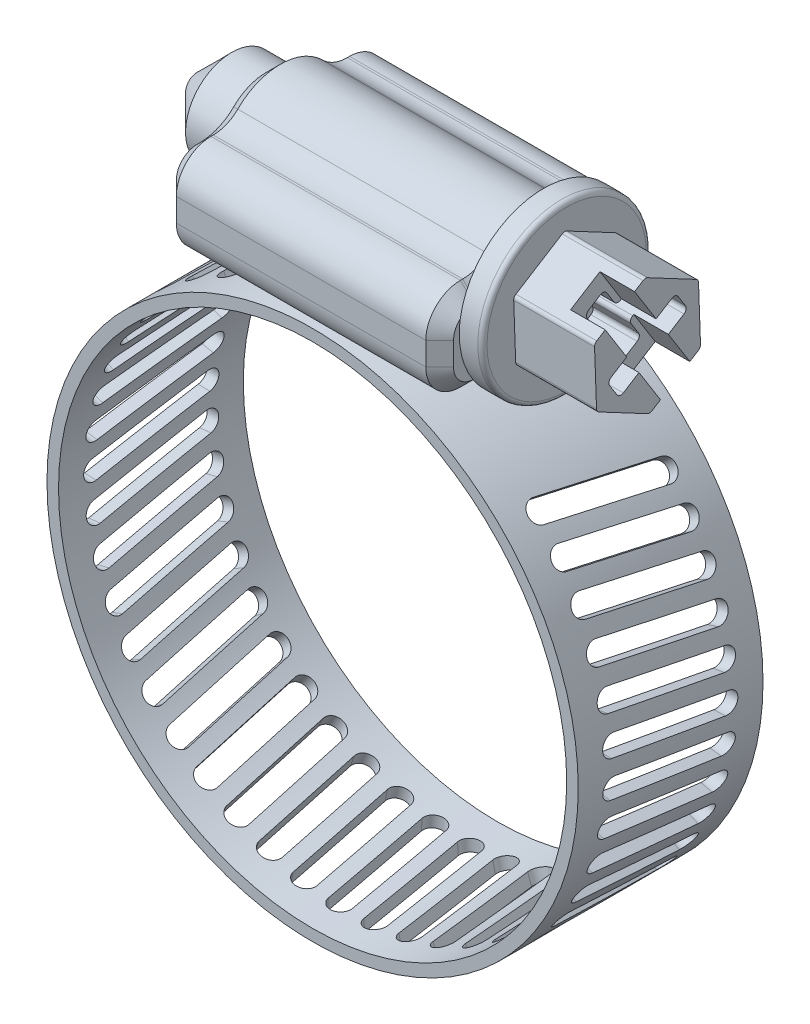
from build123d import *

# Parameters (mm, degrees)
SKETCH1_R                = 11.5
SKETCH1_R_2              = 11
EXTRUDE_THIN1_DEPTH      = 8
BOSS_EXTRUDE1_DEPTH      = 12
BOSS_EXTRUDE2_DEPTH      = 4.5
CHAMFER1_SIZE            = 0.6
FILLET1_R                = 0.2
CUT_EXTRUDE8_DEPTH       = 1.5
CUT_EXTRUDE9_DEPTH       = 2
SKETCH7_R                = 2
BOSS_EXTRUDE3_DEPTH      = 3
CHAMFER2_SIZE            = 1.5
SKETCH8_R                = 3.65
BOSS_EXTRUDE4_DEPTH      = 1
FILLET3_R                = 0.2
CUT_EXTRUDE10_REACH      = 29.083
CUT_EXTRUDE10_END_RADIUS = 11
CIRPATTERN1_COUNT        = 40
CIRPATTERN1_ANGLE        = 312


with BuildPart() as part:
    # Sketch1 → Extrude-Thin1 (new body)
    with BuildSketch(Plane.XY):
        Circle(SKETCH1_R)
        Circle(SKETCH1_R_2, mode=Mode.SUBTRACT)
    extrude(amount=EXTRUDE_THIN1_DEPTH)

    # Cut-Extrude10: up to this cylinder (the profile starts outside it)
    cut_extrude10_end = Plane(origin=(0, 0, 4), z_dir=(0, 0, -1)) * Cylinder(CUT_EXTRUDE10_END_RADIUS, 81.166, mode=Mode.PRIVATE)
    # Sketch9 → Cut-Extrude10 (cut, up to the surface)
    with BuildSketch(Plane.XZ.offset(-11.5), mode=Mode.PRIVATE) as cut_extrude10_sk1:
        with BuildLine():
            Line((-0.009043045, 1.459838938), (-0.877283933, 6.383877703))
            ThreePointArc((-0.877283933, 6.383877703), (-0.512262124, 6.905182871), (0.009043045, 6.540161062))
            Line((0.009043045, 6.540161062), (0.877283933, 1.616122297))
            ThreePointArc((0.877283933, 1.616122297), (0.512262124, 1.094817129), (-0.009043045, 1.459838938))
        make_face()
    cut_extrude10_tool1 = extrude(cut_extrude10_sk1.sketch, amount=CUT_EXTRUDE10_REACH, mode=Mode.PRIVATE) - cut_extrude10_end
    cut_extrude10 = cut_extrude10_tool1.solids().sort_by_distance((0, 11.5, 4))[0]
    add(cut_extrude10, mode=Mode.SUBTRACT)

    # CirPattern1: Cut-Extrude10 ×40 about axis
    cirpattern1_axis = Axis((0, 0, 0), (0, 0, 1))
    for i in range(1, CIRPATTERN1_COUNT):
        add(cut_extrude10.rotate(cirpattern1_axis, i * CIRPATTERN1_ANGLE / (CIRPATTERN1_COUNT - 1)), mode=Mode.SUBTRACT)


with BuildPart() as body_2:
    # Sketch2 → Boss-Extrude1 (new body)
    with BuildSketch(Plane(origin=(6, 0, 0), x_dir=(0, 0, -1), z_dir=(1, 0, 0))):
        with BuildLine():
            Line((-7, 11.5), (-1, 11.5))
            ThreePointArc((-1, 11.5), (0.060660172, 11.939339828), (0.5, 13))
            Line((0.5, 13), (0.5, 14))
            ThreePointArc((0.5, 14), (0.060660172, 15.060660172), (-1, 15.5))
            Line((-1, 15.5), (-1.1, 15.5))
            ThreePointArc((-1.1, 15.5), (-1.674110492, 15.614216055), (-2.160790803, 15.939470476))
            ThreePointArc((-2.160790803, 15.939470476), (-4, 16.701428571), (-5.839209197, 15.939470476))
            ThreePointArc((-5.839209197, 15.939470476), (-6.325889508, 15.614216055), (-6.9, 15.5))
            Line((-6.9, 15.5), (-7, 15.5))
            ThreePointArc((-7, 15.5), (-8.060660172, 15.060660172), (-8.5, 14))
            Line((-8.5, 14), (-8.5, 13))
            ThreePointArc((-8.5, 13), (-8.060660172, 11.939339828), (-7, 11.5))
        make_face()
    extrude(amount=-BOSS_EXTRUDE1_DEPTH)

    # Chamfer1
    chamfer1_edges = [body_2.edges().sort_by_distance(p)[0] for p in [
        (6, 11.5, 4),
        (6, 11.939339828, 8.060660172),
        (-6, 15.060660172, -0.060660172),
        (6, 13.5, 8.5),
        (6, 15.060660172, 8.060660172),
        (6, 15.5, 6.95),
        (6, 15.614216055, 6.325889508),
        (6, 16.701428571, 4),
        (6, 15.614216055, 1.674110492),
        (6, 15.5, 1.05),
        (6, 15.060660172, -0.060660172),
        (6, 13.5, -0.5),
        (6, 11.939339828, -0.060660172),
        (-6, 15.5, 1.05),
        (-6, 15.614216055, 1.674110492),
        (-6, 16.701428571, 4),
        (-6, 15.614216055, 6.325889508),
        (-6, 15.5, 6.95),
        (-6, 15.060660172, 8.060660172),
        (-6, 13.5, 8.5),
        (-6, 11.939339828, 8.060660172),
        (-6, 11.5, 4),
        (-6, 11.939339828, -0.060660172),
        (-6, 13.5, -0.5),
    ]]
    chamfer(chamfer1_edges, length=CHAMFER1_SIZE)

    # Sketch7 → Boss-Extrude3 (add)
    with BuildSketch(Plane.ZY.offset(6)):
        with Locations((4, 14.100714286)):
            Circle(SKETCH7_R)
    extrude(amount=BOSS_EXTRUDE3_DEPTH)

    # Chamfer2
    chamfer2_edges = [body_2.edges().sort_by_distance(p)[0] for p in [
        (-9, 14.100714286, 2),
    ]]
    chamfer(chamfer2_edges, length=CHAMFER2_SIZE)



with BuildPart() as body_3:
    # Sketch3 → Boss-Extrude2 (new body)
    with BuildSketch(Plane(origin=(6, 0, 0), x_dir=(0, 0, -1), z_dir=(1, 0, 0))):
        Polygon((-4.093468261, 16.699748429), (-6.297563724, 15.319285469), (-6.204095463, 12.720251325), (-3.906531739, 11.501680142), (-1.702436276, 12.882143103), (-1.795904537, 15.481177246), align=None)
    extrude(amount=BOSS_EXTRUDE2_DEPTH)

    # Fillet1
    fillet1_edges = [body_3.edges().sort_by_distance(p)[0] for p in [
        (8.25, 15.481177246, 1.795904537),
        (8.25, 12.882143103, 1.702436276),
        (8.25, 11.501680142, 3.906531739),
        (8.25, 12.720251325, 6.204095463),
        (8.25, 15.319285469, 6.297563724),
        (8.25, 16.699748429, 4.093468261),
    ]]
    fillet(fillet1_edges, radius=FILLET1_R)

    # Sketch5 → Cut-Extrude8 (cut)
    with BuildSketch(Plane(origin=(10.5, 0, 0), x_dir=(0, 0, -1), z_dir=(1, 0, 0))):
        with BuildLine():
            Line((-5.83113814, 15.611415848), (-4.901022881, 14.126361283))
            Line((-4.901022881, 14.126361283), (-5.579019837, 13.701720108))
            ThreePointArc((-5.579019837, 13.701720108), (-5.667780269, 13.577008267), (-5.642358783, 13.426060575))
            Line((-5.642358783, 13.426060575), (-5.323877902, 12.917562858))
            ThreePointArc((-5.323877902, 12.917562858), (-5.199166061, 12.828802427), (-5.048218369, 12.854223913))
            Line((-5.048218369, 12.854223913), (-4.370221413, 13.278865087))
            Line((-4.370221413, 13.278865087), (-3.440106154, 11.793810521))
            Line((-3.440106154, 11.793810521), (-2.16886186, 12.590012723))
            Line((-2.16886186, 12.590012723), (-3.098977119, 14.075067289))
            Line((-3.098977119, 14.075067289), (-2.420980163, 14.499708463))
            ThreePointArc((-2.420980163, 14.499708463), (-2.332219731, 14.624420304), (-2.357641217, 14.775367996))
            Line((-2.357641217, 14.775367996), (-2.676122098, 15.283865713))
            ThreePointArc((-2.676122098, 15.283865713), (-2.800833939, 15.372626145), (-2.951781631, 15.347204659))
            Line((-2.951781631, 15.347204659), (-3.629778587, 14.922563484))
            Line((-3.629778587, 14.922563484), (-4.559893846, 16.40761805))
            Line((-4.559893846, 16.40761805), (-5.83113814, 15.611415848))
        make_face()
    extrude(amount=-CUT_EXTRUDE8_DEPTH, mode=Mode.SUBTRACT)

    # Sketch6 → Cut-Extrude9 (cut)
    with BuildSketch(Plane(origin=(9, 0, 0), x_dir=(0, 0, -1), z_dir=(1, 0, 0))):
        with BuildLine():
            Line((-2.951781631, 15.347204659), (-3.672153397, 14.896023411))
            ThreePointArc((-3.672153397, 14.896023411), (-3.823101089, 14.870601925), (-3.94781293, 14.959362357))
            Line((-3.94781293, 14.959362357), (-4.266293811, 15.467860074))
            ThreePointArc((-4.266293811, 15.467860074), (-4.391005652, 15.556620505), (-4.541953343, 15.53119902))
            Line((-4.541953343, 15.53119902), (-5.050451061, 15.212718139))
            ThreePointArc((-5.050451061, 15.212718139), (-5.139211492, 15.088006298), (-5.113790006, 14.937058606))
            Line((-5.113790006, 14.937058606), (-4.795309125, 14.428560889))
            ThreePointArc((-4.795309125, 14.428560889), (-4.76988764, 14.277613197), (-4.858648071, 14.152901356))
            Line((-4.858648071, 14.152901356), (-5.579019837, 13.701720108))
            ThreePointArc((-5.579019837, 13.701720108), (-5.667780269, 13.577008267), (-5.642358783, 13.426060575))
            Line((-5.642358783, 13.426060575), (-5.323877902, 12.917562858))
            ThreePointArc((-5.323877902, 12.917562858), (-5.199166061, 12.828802427), (-5.048218369, 12.854223913))
            Line((-5.048218369, 12.854223913), (-4.327846603, 13.30540516))
            ThreePointArc((-4.327846603, 13.30540516), (-4.176898911, 13.330826646), (-4.05218707, 13.242066215))
            Line((-4.05218707, 13.242066215), (-3.733706189, 12.733568497))
            ThreePointArc((-3.733706189, 12.733568497), (-3.608994348, 12.644808066), (-3.458046657, 12.670229552))
            Line((-3.458046657, 12.670229552), (-2.949548939, 12.988710433))
            ThreePointArc((-2.949548939, 12.988710433), (-2.860788508, 13.113422274), (-2.886209994, 13.264369965))
            Line((-2.886209994, 13.264369965), (-3.204690875, 13.772867683))
            ThreePointArc((-3.204690875, 13.772867683), (-3.23011236, 13.923815374), (-3.141351929, 14.048527215))
            Line((-3.141351929, 14.048527215), (-2.420980163, 14.499708463))
            ThreePointArc((-2.420980163, 14.499708463), (-2.332219731, 14.624420304), (-2.357641217, 14.775367996))
            Line((-2.357641217, 14.775367996), (-2.676122098, 15.283865713))
            ThreePointArc((-2.676122098, 15.283865713), (-2.800833939, 15.372626145), (-2.951781631, 15.347204659))
        make_face()
    extrude(amount=-CUT_EXTRUDE9_DEPTH, mode=Mode.SUBTRACT)


with BuildPart() as body_2_1:
    add(body_2.part)

    add(body_3.part)  # Boss-Extrude4 merges body 3
    # Sketch8 → Boss-Extrude4 (add)
    with BuildSketch(Plane.ZY.offset(-6)):
        with Locations((4, 14.100714286)):
            Circle(SKETCH8_R)
    extrude(amount=-BOSS_EXTRUDE4_DEPTH)

    # Fillet3
    fillet3_edges = [body_2_1.edges().sort_by_distance(p)[0] for p in [
        (7, 14.100714286, 0.35),
    ]]
    fillet(fillet3_edges, radius=FILLET3_R)


solid = Compound([part.part, body_2_1.part])
